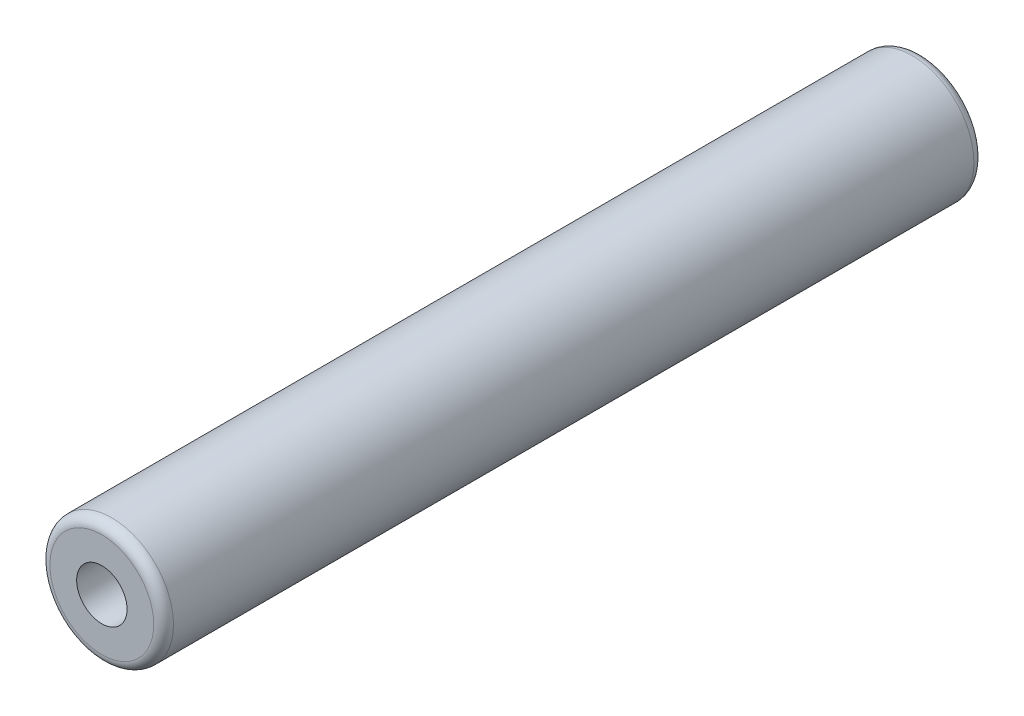
from build123d import *

# Parameters (mm, degrees)
SKETCH1_R              = 12.5
BOSS_EXTRUDE1_DEPTH    = 166
FILLET1_R              = 2
M12_TAPPED_HOLE1_D     = 10.2
M12_TAPPED_HOLE1_DEPTH = 30
M12_TAPPED_HOLE1_TIP   = 3.064389157
M12_TAPPED_HOLE2_D     = 10.2
M12_TAPPED_HOLE2_DEPTH = 30
M12_TAPPED_HOLE2_TIP   = 3.064389157


with BuildPart() as part:
    # Sketch1 → Boss-Extrude1 (new body)
    with BuildSketch(Plane.XY):
        Circle(SKETCH1_R)
    extrude(amount=BOSS_EXTRUDE1_DEPTH)

    # Fillet1
    fillet1_edges = [part.edges().sort_by_distance(p)[0] for p in [
        (-12.5, 0, 0),
        (-12.5, 0, 166),
    ]]
    fillet(fillet1_edges, radius=FILLET1_R)

    # M12 Tapped Hole1
    with Locations(Plane.XY.offset(166)):
        with Locations((0, 0)):
            Hole(M12_TAPPED_HOLE1_D / 2, depth=M12_TAPPED_HOLE1_DEPTH)
            with Locations((0, 0, -(M12_TAPPED_HOLE1_DEPTH + M12_TAPPED_HOLE1_TIP / 2))):  # 118° drill point
                Cone(0, M12_TAPPED_HOLE1_D / 2, M12_TAPPED_HOLE1_TIP, mode=Mode.SUBTRACT)

    # M12 Tapped Hole2
    with Locations(Plane(origin=(0, 0, 0), x_dir=(-1, 0, 0), z_dir=(0, 0, -1))):
        with Locations((0, 0)):
            Hole(M12_TAPPED_HOLE2_D / 2, depth=M12_TAPPED_HOLE2_DEPTH)
            with Locations((0, 0, -(M12_TAPPED_HOLE2_DEPTH + M12_TAPPED_HOLE2_TIP / 2))):  # 118° drill point
                Cone(0, M12_TAPPED_HOLE2_D / 2, M12_TAPPED_HOLE2_TIP, mode=Mode.SUBTRACT)


solid = part.part
